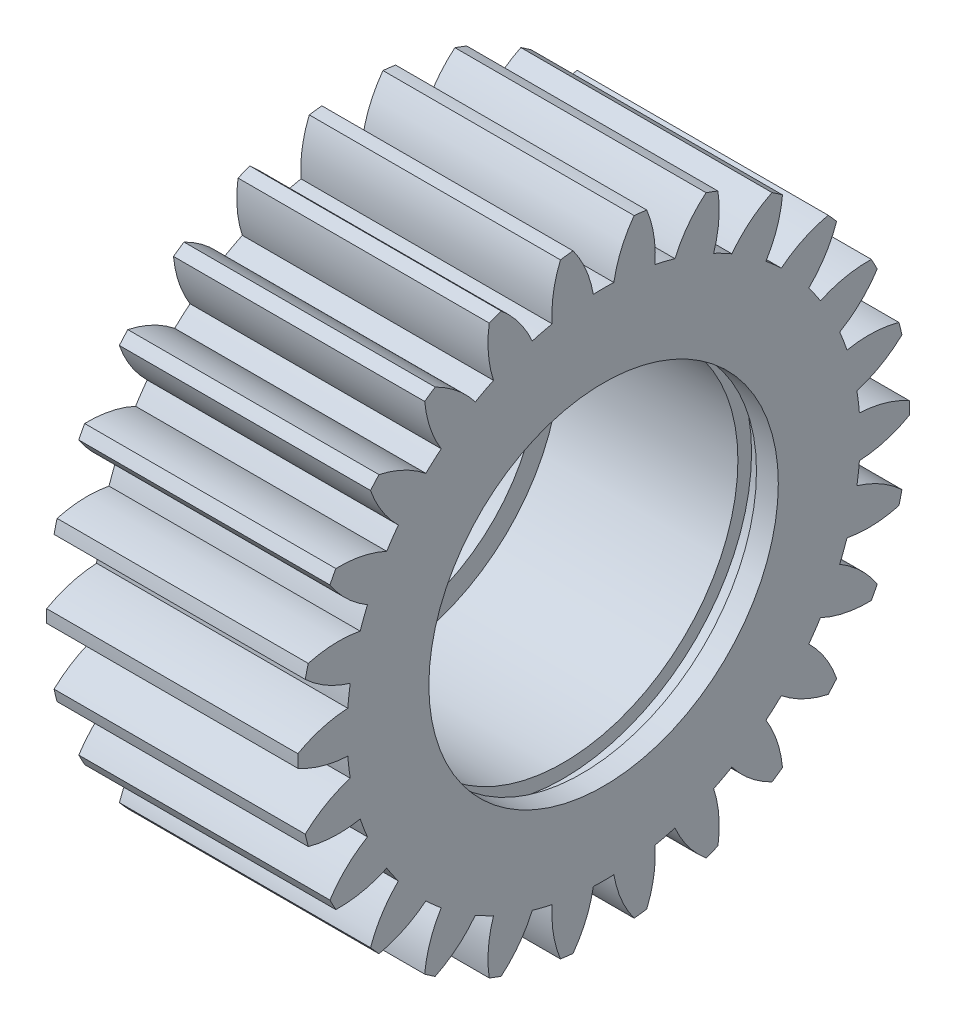
from build123d import *

# Parameters (mm, degrees)
SKETCH_1_W           = 23
SKETCH_1_H           = 28
CUT_EXTRUDE_1_DEPTH  = 46.793012567
CUT_EXTRUDE_2_DEPTH  = 46.793012567
CUT_EXTRUDE_3_DEPTH  = 46.793012567
CUT_EXTRUDE_4_DEPTH  = 46.793012567
CUT_EXTRUDE_5_DEPTH  = 46.793012567
CUT_EXTRUDE_6_DEPTH  = 46.793012567
CUT_EXTRUDE_7_DEPTH  = 46.793012567
CUT_EXTRUDE_8_DEPTH  = 46.793012567
CUT_EXTRUDE_9_DEPTH  = 46.793012567
CUT_EXTRUDE_10_DEPTH = 46.793012567
CUT_EXTRUDE_11_DEPTH = 46.793012567
CUT_EXTRUDE_12_DEPTH = 46.793012567
CUT_EXTRUDE_13_DEPTH = 46.793012567
CUT_EXTRUDE_14_DEPTH = 46.793012567
CUT_EXTRUDE_15_DEPTH = 46.793012567
CUT_EXTRUDE_16_DEPTH = 46.793012567
CUT_EXTRUDE_17_DEPTH = 46.793012567
CUT_EXTRUDE_18_DEPTH = 46.793012567
CUT_EXTRUDE_19_DEPTH = 46.793012567
CUT_EXTRUDE_20_DEPTH = 46.793012567
CUT_EXTRUDE_21_DEPTH = 46.793012567
CUT_EXTRUDE_22_DEPTH = 46.793012567
CUT_EXTRUDE_23_DEPTH = 46.707554998
CUT_EXTRUDE_24_DEPTH = 46.707554998
CUT_EXTRUDE_25_DEPTH = 46.707554998
CUT_EXTRUDE_26_DEPTH = 46.707554998


with BuildPart() as part:
    # 草图1 → 旋转1 (revolve)
    with BuildSketch(Plane(origin=(0, 0, 0), x_dir=(-1, 0, 0), z_dir=(0, 0, -1)), mode=Mode.PRIVATE) as revolve_1_sk:
        with Locations((-8.5, 14)):
            Rectangle(SKETCH_1_W, SKETCH_1_H)
    revolve(revolve_1_sk.sketch.rotate(Axis((20, 0, 0), (-1, 0, 0)), 270), axis=Axis((20, 0, 0), (-1, 0, 0)))

    # 草图2 → 切除-拉伸1 (cut, through all)
    with BuildSketch(Plane.ZY.offset(3)):
        with BuildLine():
            ThreePointArc((27.04115844, 7.264692024), (26.180454795, 9.928936837), (25.057979622, 12.493904805))
            ThreePointArc((25.057979622, 12.493904805), (23.530106712, 10.650293105), (21.621088432, 9.20497344))
            ThreePointArc((21.621088432, 9.20497344), (21.971946687, 8.332860241), (22.287643535, 7.447412078))
            ThreePointArc((22.287643535, 7.447412078), (24.674988454, 7.631488051), (27.04115844, 7.264692024))
        make_face()
    extrude(amount=-CUT_EXTRUDE_1_DEPTH, mode=Mode.SUBTRACT)

    # 草图3 → 切除-拉伸2 (cut, through all)
    with BuildSketch(Plane.ZY.offset(3)):
        with BuildLine():
            ThreePointArc((27.993946119, 0.582220482), (27.795848475, 3.375027047), (27.319827403, 6.134087599))
            ThreePointArc((27.319827403, 6.134087599), (25.395146544, 4.709691825), (23.19571323, 3.763228501))
            ThreePointArc((23.19571323, 3.763228501), (23.327665832, 2.832491449), (23.422287489, 1.897221601))
            ThreePointArc((23.422287489, 1.897221601), (25.784312767, 1.504619625), (27.993946119, 0.582220482))
        make_face()
    extrude(amount=-CUT_EXTRUDE_2_DEPTH, mode=Mode.SUBTRACT)

    # 草图4 → 切除-拉伸3 (cut, through all)
    with BuildSketch(Plane.ZY.offset(3)):
        with BuildLine():
            ThreePointArc((27.319827403, -6.134087599), (27.795848475, -3.375027047), (27.993946119, -0.582220482))
            ThreePointArc((27.993946119, -0.582220482), (25.784312767, -1.504619625), (23.422287489, -1.897221601))
            ThreePointArc((23.422287489, -1.897221601), (23.327665832, -2.832491449), (23.19571323, -3.763228501))
            ThreePointArc((23.19571323, -3.763228501), (25.395146544, -4.709691825), (27.319827403, -6.134087599))
        make_face()
    extrude(amount=-CUT_EXTRUDE_3_DEPTH, mode=Mode.SUBTRACT)

    # 草图5 → 切除-拉伸4 (cut, through all)
    with BuildSketch(Plane.ZY.offset(3)):
        with BuildLine():
            ThreePointArc((25.057979622, -12.493904805), (26.180454795, -9.928936837), (27.04115844, -7.264692024))
            ThreePointArc((27.04115844, -7.264692024), (24.674988454, -7.631488051), (22.287643535, -7.447412078))
            ThreePointArc((22.287643535, -7.447412078), (21.971946687, -8.332860241), (21.621088432, -9.20497344))
            ThreePointArc((21.621088432, -9.20497344), (23.530106712, -10.650293105), (25.057979622, -12.493904805))
        make_face()
    extrude(amount=-CUT_EXTRUDE_4_DEPTH, mode=Mode.SUBTRACT)

    # 草图6 → 切除-拉伸5 (cut, through all)
    with BuildSketch(Plane.ZY.offset(3)):
        with BuildLine():
            ThreePointArc((21.339853147, -18.127621677), (23.043548245, -15.905812908), (24.516836924, -13.524966072))
            ThreePointArc((24.516836924, -13.524966072), (22.131643502, -13.314842131), (19.857722751, -12.564786036))
            ThreePointArc((19.857722751, -12.564786036), (19.339297865, -13.348953483), (18.789924563, -14.111758782))
            ThreePointArc((18.789924563, -14.111758782), (20.297582605, -15.971938062), (21.339853147, -18.127621677))
        make_face()
    extrude(amount=-CUT_EXTRUDE_5_DEPTH, mode=Mode.SUBTRACT)

    # 草图7 → 切除-拉伸6 (cut, through all)
    with BuildSketch(Plane.ZY.offset(3)):
        with BuildLine():
            ThreePointArc((16.381531975, -22.707827068), (18.567434431, -20.958300949), (20.56768596, -18.999218253))
            ThreePointArc((20.56768596, -18.999218253), (18.302087875, -18.224385984), (16.273743301, -16.951940301))
            ThreePointArc((16.273743301, -16.951940301), (15.582719346, -17.589254071), (14.866758577, -18.198419997))
            ThreePointArc((14.866758577, -18.198419997), (15.885436777, -20.365352035), (16.381531975, -22.707827068))
        make_face()
    extrude(amount=-CUT_EXTRUDE_6_DEPTH, mode=Mode.SUBTRACT)

    # 草图8 → 切除-拉伸7 (cut, through all)
    with BuildSketch(Plane.ZY.offset(3)):
        with BuildLine():
            ThreePointArc((15.423215849, -23.369304929), (13.408881426, -22.074794766), (11.743993043, -20.353909413))
            ThreePointArc((11.743993043, -20.353909413), (10.92052982, -20.807331147), (10.079590622, -21.227455191))
            ThreePointArc((10.079590622, -21.227455191), (10.550087104, -23.575205772), (10.471175709, -25.96833609))
            ThreePointArc((10.471175709, -25.96833609), (13.012248817, -24.792768718), (15.423215849, -23.369304929))
        make_face()
    extrude(amount=-CUT_EXTRUDE_7_DEPTH, mode=Mode.SUBTRACT)

    # 草图9 → 切除-拉伸8 (cut, through all)
    with BuildSketch(Plane.ZY.offset(3)):
        with BuildLine():
            ThreePointArc((9.382404494, -26.381252546), (7.736399528, -24.642296716), (6.531724597, -22.572983294))
            ThreePointArc((6.531724597, -22.572983294), (5.623678795, -22.816161768), (4.706633497, -23.022827848))
            ThreePointArc((4.706633497, -23.022827848), (4.601604717, -25.414954242), (3.952272771, -27.719659809))
            ThreePointArc((3.952272771, -27.719659809), (6.7008386, -27.186370888), (9.382404494, -26.381252546))
        make_face()
    extrude(amount=-CUT_EXTRUDE_8_DEPTH, mode=Mode.SUBTRACT)

    # 草图10 → 切除-拉伸9 (cut, through all)
    with BuildSketch(Plane.ZY.offset(3)):
        with BuildLine():
            ThreePointArc((-2.796321894, -27.860017657), (0, -28), (2.796321894, -27.860017657))
            ThreePointArc((2.796321894, -27.860017657), (1.61430621, -25.777677951), (0.939856059, -23.480197435))
            ThreePointArc((0.939856059, -23.480197435), (0, -23.499), (-0.939856059, -23.480197435))
            ThreePointArc((-0.939856059, -23.480197435), (-1.61430621, -25.777677951), (-2.796321894, -27.860017657))
        make_face()
    extrude(amount=-CUT_EXTRUDE_9_DEPTH, mode=Mode.SUBTRACT)

    # 草图11 → 切除-拉伸10 (cut, through all)
    with BuildSketch(Plane.ZY.offset(3)):
        with BuildLine():
            ThreePointArc((-9.382404494, -26.381252546), (-6.7008386, -27.186370888), (-3.952272771, -27.719659809))
            ThreePointArc((-3.952272771, -27.719659809), (-4.601604717, -25.414954242), (-4.706633497, -23.022827848))
            ThreePointArc((-4.706633497, -23.022827848), (-5.623678795, -22.816161768), (-6.531724597, -22.572983294))
            ThreePointArc((-6.531724597, -22.572983294), (-7.736399528, -24.642296716), (-9.382404494, -26.381252546))
        make_face()
    extrude(amount=-CUT_EXTRUDE_10_DEPTH, mode=Mode.SUBTRACT)

    # 草图12 → 切除-拉伸11 (cut, through all)
    with BuildSketch(Plane.ZY.offset(3)):
        with BuildLine():
            ThreePointArc((-15.423215849, -23.369304929), (-13.012248817, -24.792768718), (-10.471175709, -25.96833609))
            ThreePointArc((-10.471175709, -25.96833609), (-10.550087104, -23.575205772), (-10.079590622, -21.227455191))
            ThreePointArc((-10.079590622, -21.227455191), (-10.92052982, -20.807331147), (-11.743993043, -20.353909413))
            ThreePointArc((-11.743993043, -20.353909413), (-13.408881426, -22.074794766), (-15.423215849, -23.369304929))
        make_face()
    extrude(amount=-CUT_EXTRUDE_11_DEPTH, mode=Mode.SUBTRACT)

    # 草图13 → 切除-拉伸12 (cut, through all)
    with BuildSketch(Plane.ZY.offset(3)):
        with BuildLine():
            ThreePointArc((-20.56768596, -18.999218253), (-18.567434431, -20.958300949), (-16.381531975, -22.707827068))
            ThreePointArc((-16.381531975, -22.707827068), (-15.885436777, -20.365352035), (-14.866758577, -18.198419997))
            ThreePointArc((-14.866758577, -18.198419997), (-15.582719346, -17.589254071), (-16.273743301, -16.951940301))
            ThreePointArc((-16.273743301, -16.951940301), (-18.302087875, -18.224385984), (-20.56768596, -18.999218253))
        make_face()
    extrude(amount=-CUT_EXTRUDE_12_DEPTH, mode=Mode.SUBTRACT)

    # 草图14 → 切除-拉伸13 (cut, through all)
    with BuildSketch(Plane.ZY.offset(3)):
        with BuildLine():
            ThreePointArc((-24.516836924, -13.524966072), (-23.043548245, -15.905812908), (-21.339853147, -18.127621677))
            ThreePointArc((-21.339853147, -18.127621677), (-20.297582605, -15.971938062), (-18.789924563, -14.111758782))
            ThreePointArc((-18.789924563, -14.111758782), (-19.339297865, -13.348953483), (-19.857722751, -12.564786036))
            ThreePointArc((-19.857722751, -12.564786036), (-22.131643502, -13.314842131), (-24.516836924, -13.524966072))
        make_face()
    extrude(amount=-CUT_EXTRUDE_13_DEPTH, mode=Mode.SUBTRACT)

    # 草图15 → 切除-拉伸14 (cut, through all)
    with BuildSketch(Plane.ZY.offset(3)):
        with BuildLine():
            ThreePointArc((-27.04115844, -7.264692024), (-26.180454795, -9.928936837), (-25.057979622, -12.493904805))
            ThreePointArc((-25.057979622, -12.493904805), (-23.530106712, -10.650293105), (-21.621088432, -9.20497344))
            ThreePointArc((-21.621088432, -9.20497344), (-21.971946687, -8.332860241), (-22.287643535, -7.447412078))
            ThreePointArc((-22.287643535, -7.447412078), (-24.674988454, -7.631488051), (-27.04115844, -7.264692024))
        make_face()
    extrude(amount=-CUT_EXTRUDE_14_DEPTH, mode=Mode.SUBTRACT)

    # 草图16 → 切除-拉伸15 (cut, through all)
    with BuildSketch(Plane.ZY.offset(3)):
        with BuildLine():
            ThreePointArc((-27.993946119, -0.582220482), (-27.795848475, -3.375027047), (-27.319827403, -6.134087599))
            ThreePointArc((-27.319827403, -6.134087599), (-25.395146544, -4.709691825), (-23.19571323, -3.763228501))
            ThreePointArc((-23.19571323, -3.763228501), (-23.327665832, -2.832491449), (-23.422287489, -1.897221601))
            ThreePointArc((-23.422287489, -1.897221601), (-25.784312767, -1.504619625), (-27.993946119, -0.582220482))
        make_face()
    extrude(amount=-CUT_EXTRUDE_15_DEPTH, mode=Mode.SUBTRACT)

    # 草图17 → 切除-拉伸16 (cut, through all)
    with BuildSketch(Plane.ZY.offset(3)):
        with BuildLine():
            ThreePointArc((-27.319827403, 6.134087599), (-27.795848475, 3.375027047), (-27.993946119, 0.582220482))
            ThreePointArc((-27.993946119, 0.582220482), (-25.784312767, 1.504619625), (-23.422287489, 1.897221601))
            ThreePointArc((-23.422287489, 1.897221601), (-23.327665832, 2.832491449), (-23.19571323, 3.763228501))
            ThreePointArc((-23.19571323, 3.763228501), (-25.395146544, 4.709691825), (-27.319827403, 6.134087599))
        make_face()
    extrude(amount=-CUT_EXTRUDE_16_DEPTH, mode=Mode.SUBTRACT)

    # 草图18 → 切除-拉伸17 (cut, through all)
    with BuildSketch(Plane.ZY.offset(3)):
        with BuildLine():
            ThreePointArc((-25.057979622, 12.493904805), (-26.180454795, 9.928936837), (-27.04115844, 7.264692024))
            ThreePointArc((-27.04115844, 7.264692024), (-24.674988454, 7.631488051), (-22.287643535, 7.447412078))
            ThreePointArc((-22.287643535, 7.447412078), (-21.971946687, 8.332860241), (-21.621088432, 9.20497344))
            ThreePointArc((-21.621088432, 9.20497344), (-23.530106712, 10.650293105), (-25.057979622, 12.493904805))
        make_face()
    extrude(amount=-CUT_EXTRUDE_17_DEPTH, mode=Mode.SUBTRACT)

    # 草图19 → 切除-拉伸18 (cut, through all)
    with BuildSketch(Plane.ZY.offset(3)):
        with BuildLine():
            ThreePointArc((-21.339853147, 18.127621677), (-23.043548245, 15.905812908), (-24.516836924, 13.524966072))
            ThreePointArc((-24.516836924, 13.524966072), (-22.131643502, 13.314842131), (-19.857722751, 12.564786036))
            ThreePointArc((-19.857722751, 12.564786036), (-19.339297865, 13.348953483), (-18.789924563, 14.111758782))
            ThreePointArc((-18.789924563, 14.111758782), (-20.297582605, 15.971938062), (-21.339853147, 18.127621677))
        make_face()
    extrude(amount=-CUT_EXTRUDE_18_DEPTH, mode=Mode.SUBTRACT)

    # 草图20 → 切除-拉伸19 (cut, through all)
    with BuildSketch(Plane.ZY.offset(3)):
        with BuildLine():
            ThreePointArc((-16.381531975, 22.707827068), (-18.567434431, 20.958300949), (-20.56768596, 18.999218253))
            ThreePointArc((-20.56768596, 18.999218253), (-18.302087875, 18.224385984), (-16.273743301, 16.951940301))
            ThreePointArc((-16.273743301, 16.951940301), (-15.582719346, 17.589254071), (-14.866758577, 18.198419997))
            ThreePointArc((-14.866758577, 18.198419997), (-15.885436777, 20.365352035), (-16.381531975, 22.707827068))
        make_face()
    extrude(amount=-CUT_EXTRUDE_19_DEPTH, mode=Mode.SUBTRACT)

    # 草图21 → 切除-拉伸20 (cut, through all)
    with BuildSketch(Plane.ZY.offset(3)):
        with BuildLine():
            ThreePointArc((-10.471175709, 25.96833609), (-13.012248817, 24.792768718), (-15.423215849, 23.369304929))
            ThreePointArc((-15.423215849, 23.369304929), (-13.408881426, 22.074794766), (-11.743993043, 20.353909413))
            ThreePointArc((-11.743993043, 20.353909413), (-10.92052982, 20.807331147), (-10.079590622, 21.227455191))
            ThreePointArc((-10.079590622, 21.227455191), (-10.550087104, 23.575205772), (-10.471175709, 25.96833609))
        make_face()
    extrude(amount=-CUT_EXTRUDE_20_DEPTH, mode=Mode.SUBTRACT)

    # 草图22 → 切除-拉伸21 (cut, through all)
    with BuildSketch(Plane.ZY.offset(3)):
        with BuildLine():
            ThreePointArc((-3.952272771, 27.719659809), (-6.7008386, 27.186370888), (-9.382404494, 26.381252546))
            ThreePointArc((-9.382404494, 26.381252546), (-7.736399528, 24.642296716), (-6.531724597, 22.572983294))
            ThreePointArc((-6.531724597, 22.572983294), (-5.623678795, 22.816161768), (-4.706633497, 23.022827848))
            ThreePointArc((-4.706633497, 23.022827848), (-4.601604717, 25.414954242), (-3.952272771, 27.719659809))
        make_face()
    extrude(amount=-CUT_EXTRUDE_21_DEPTH, mode=Mode.SUBTRACT)

    # 草图23 → 切除-拉伸22 (cut, through all)
    with BuildSketch(Plane.ZY.offset(3)):
        with BuildLine():
            ThreePointArc((2.796321894, 27.860017657), (0, 28), (-2.796321894, 27.860017657))
            ThreePointArc((-2.796321894, 27.860017657), (-1.61430621, 25.777677951), (-0.939856059, 23.480197435))
            ThreePointArc((-0.939856059, 23.480197435), (0, 23.499), (0.939856059, 23.480197435))
            ThreePointArc((0.939856059, 23.480197435), (1.61430621, 25.777677951), (2.796321894, 27.860017657))
        make_face()
    extrude(amount=-CUT_EXTRUDE_22_DEPTH, mode=Mode.SUBTRACT)

    # 草图24 → 切除-拉伸23 (cut, through all)
    with BuildSketch(Plane.ZY.offset(3)):
        with BuildLine():
            ThreePointArc((9.382404494, 26.381252546), (6.7008386, 27.186370888), (3.952272771, 27.719659809))
            ThreePointArc((3.952272771, 27.719659809), (4.601604717, 25.414954242), (4.706633497, 23.022827848))
            ThreePointArc((4.706633497, 23.022827848), (5.623678795, 22.816161768), (6.531724597, 22.572983294))
            ThreePointArc((6.531724597, 22.572983294), (7.736399528, 24.642296716), (9.382404494, 26.381252546))
        make_face()
    extrude(amount=-CUT_EXTRUDE_23_DEPTH, mode=Mode.SUBTRACT)

    # 草图25 → 切除-拉伸24 (cut, through all)
    with BuildSketch(Plane.ZY.offset(3)):
        with BuildLine():
            ThreePointArc((15.423215849, 23.369304929), (13.012248817, 24.792768718), (10.471175709, 25.96833609))
            ThreePointArc((10.471175709, 25.96833609), (10.550087104, 23.575205772), (10.079590622, 21.227455191))
            ThreePointArc((10.079590622, 21.227455191), (10.92052982, 20.807331147), (11.743993043, 20.353909413))
            ThreePointArc((11.743993043, 20.353909413), (13.408881426, 22.074794766), (15.423215849, 23.369304929))
        make_face()
    extrude(amount=-CUT_EXTRUDE_24_DEPTH, mode=Mode.SUBTRACT)

    # 草图26 → 切除-拉伸25 (cut, through all)
    with BuildSketch(Plane.ZY.offset(3)):
        with BuildLine():
            ThreePointArc((20.56768596, 18.999218253), (18.567434431, 20.958300949), (16.381531975, 22.707827068))
            ThreePointArc((16.381531975, 22.707827068), (15.885436777, 20.365352035), (14.866758577, 18.198419997))
            ThreePointArc((14.866758577, 18.198419997), (15.582719346, 17.589254071), (16.273743301, 16.951940301))
            ThreePointArc((16.273743301, 16.951940301), (18.302087875, 18.224385984), (20.56768596, 18.999218253))
        make_face()
    extrude(amount=-CUT_EXTRUDE_25_DEPTH, mode=Mode.SUBTRACT)

    # 草图27 → 切除-拉伸26 (cut, through all)
    with BuildSketch(Plane.ZY.offset(3)):
        with BuildLine():
            ThreePointArc((24.516836924, 13.524966072), (23.043548245, 15.905812908), (21.339853147, 18.127621677))
            ThreePointArc((21.339853147, 18.127621677), (20.297582605, 15.971938062), (18.789924563, 14.111758782))
            ThreePointArc((18.789924563, 14.111758782), (19.339297865, 13.348953483), (19.857722751, 12.564786036))
            ThreePointArc((19.857722751, 12.564786036), (22.131643502, 13.314842131), (24.516836924, 13.524966072))
        make_face()
    extrude(amount=-CUT_EXTRUDE_26_DEPTH, mode=Mode.SUBTRACT)

    # 草图28 → 切除-旋转1 (revolve, cut)
    with BuildSketch(Plane.XY, mode=Mode.PRIVATE) as cut_revolve_1_sk:
        Polygon((-3, 14), (-3, 0), (20, 0), (20, 16), (18, 16), (18, 17.25), (16.3, 17.25), (16.3, 16), (0, 16), (0, 14), align=None)
    revolve(cut_revolve_1_sk.sketch.rotate(Axis((-3, 0, 0), (1, 0, 0)), 270), axis=Axis((-3, 0, 0), (1, 0, 0)), mode=Mode.SUBTRACT)


solid = part.part
